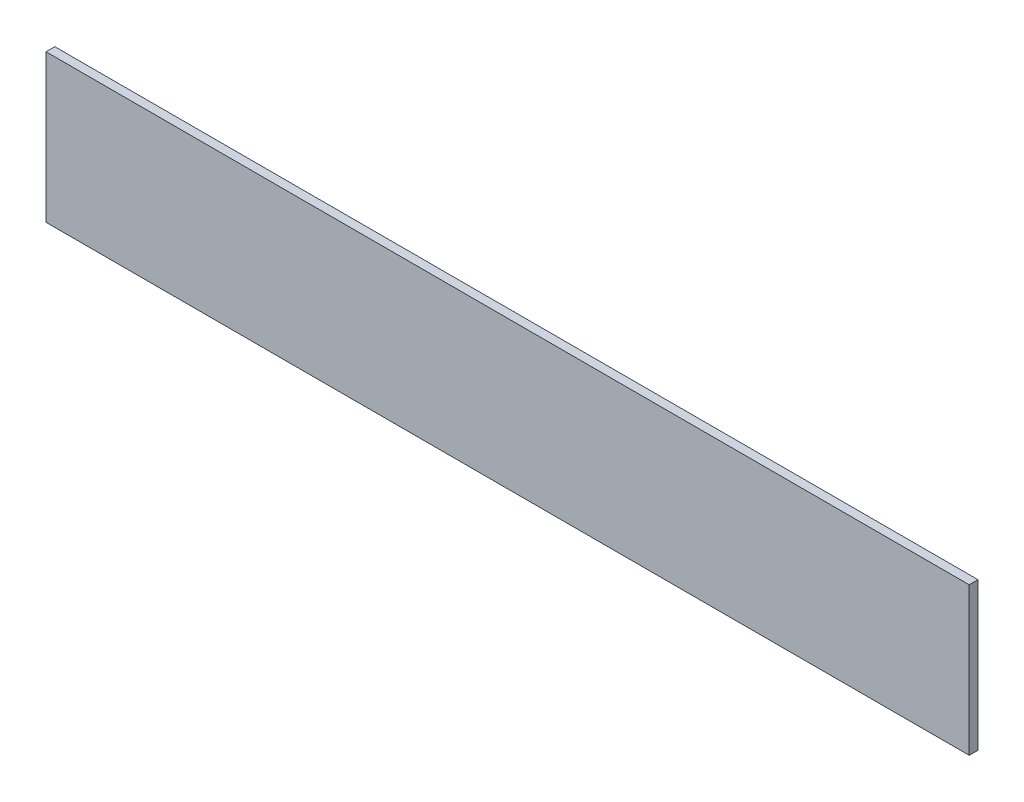
from build123d import *

# Parameters (mm, degrees)
SKETCH1_W           = 2100
SKETCH1_H           = 336
BOSS_EXTRUDE1_DEPTH = 10


with BuildPart() as part:
    # Sketch1 → Boss-Extrude1 (new, symmetric)
    with BuildSketch(Plane.XY):
        Rectangle(SKETCH1_W, SKETCH1_H)
    extrude(amount=BOSS_EXTRUDE1_DEPTH, both=True)


solid = part.part
